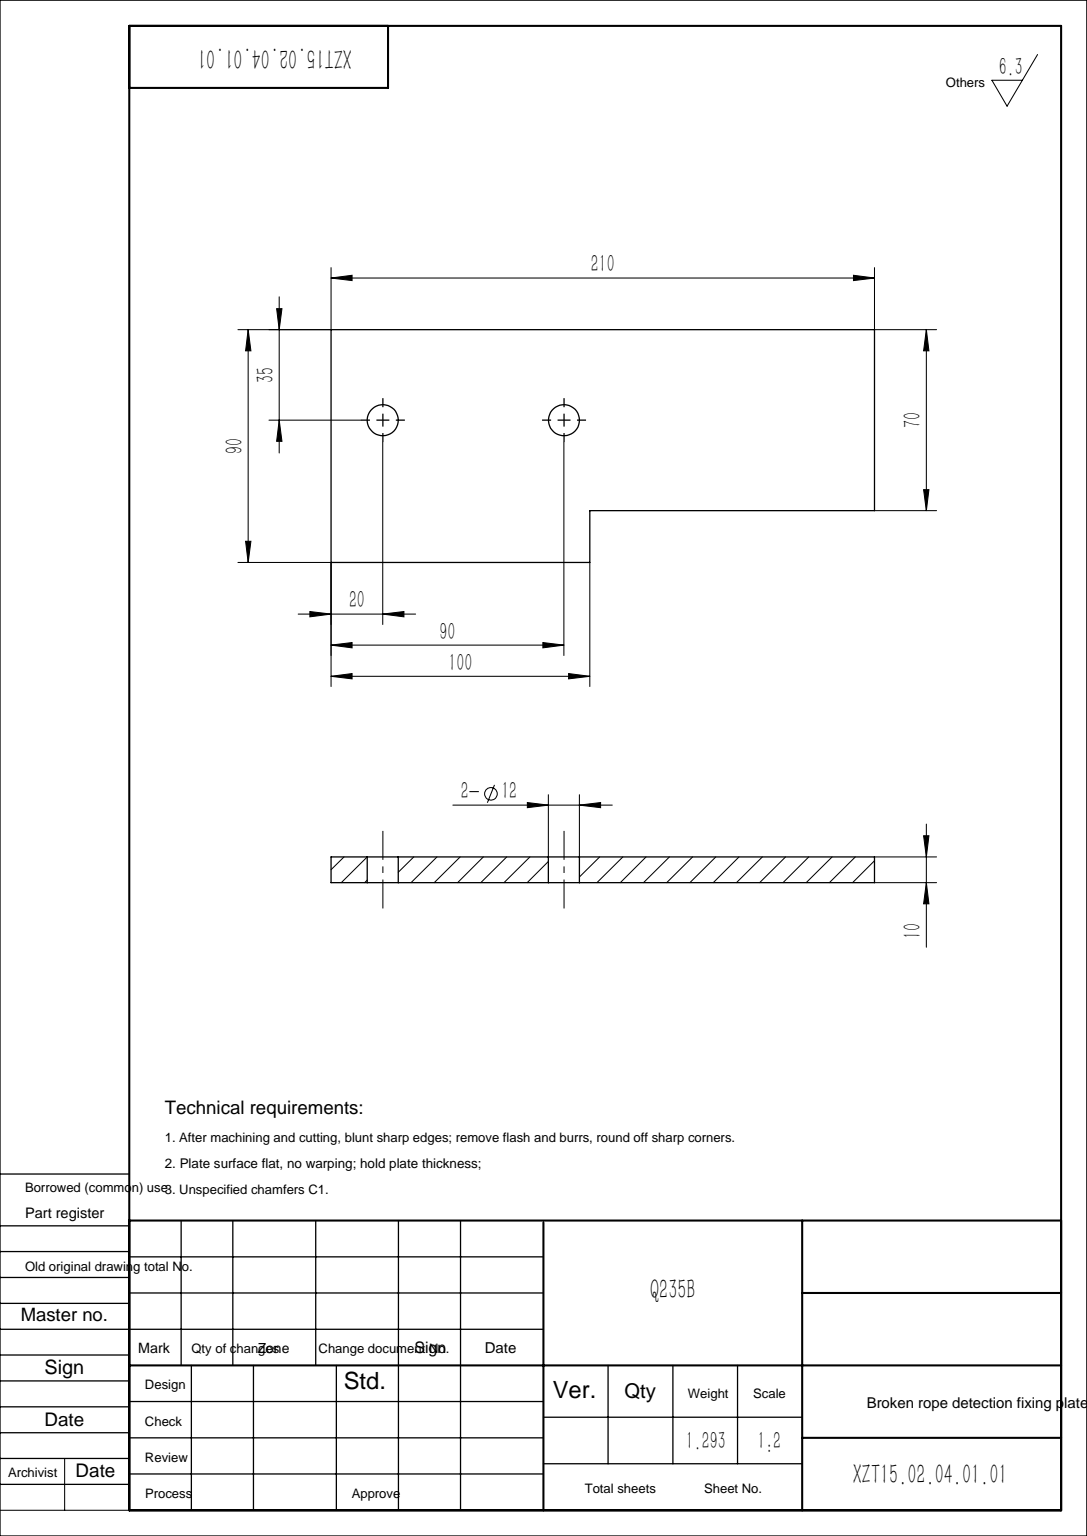
SolidWorks part; units mm, degrees
material "Q235B"
ref_plane "Front Plane" through (0, 0, 0) normal (0, 0, 1) x (1, 0, 0)
ref_plane "Top Plane" through (0, 0, 0) normal (0, 1, 0) x (1, 0, 0)
ref_plane "Right Plane" through (0, 0, 0) normal (1, 0, 0) x (0, 0, -1)
sketch "Sketch1" plane through (0, 0, 0) normal (0, 0, 1) x (1, 0, 0)
  line L0 (0, 0) -> (0, 90)
  line L1 (0, 90) -> (210, 90)
  line L2 (210, 90) -> (210, 20)
  line L3 (210, 20) -> (100, 20)
  line L4 (100, 20) -> (100, 0)
  line L5 (100, 0) -> (0, 0)
  dimension "D1" = 100
  dimension "D2" = 70
  dimension "D3" = 210
  dimension "D4" = 90
extrude "Boss-Extrude1" add sketch "Sketch1" along normal mid plane 10
hole_wizard "Ø12.0 (12) Diameter Hole1" positions "Sketch2" profile "Sketch3" hole size "Ø12.0" standard "GB" end condition up to next
sketch "Sketch2" plane through (0, 0, 5) normal (0, 0, 1) x (1, 0, 0)
  line L0 (210, 90) -> (0, 90) construction
  line L1 (0, 90) -> (0, 0) construction
  point P0 (20, 55)
  point P2 (90, 55)
  dimension "D1" = 35
  dimension "D2" = 20
  dimension "D3" = 90
sketch "Sketch3" plane through (20, 55, 5) normal (1, 0, 0) x (0, -1, 0)
  line L0 (0, 0) -> (0, 10)
  line L1 (0, 10) -> (6, 10)
  line L2 (6, 10) -> (6, 0)
  line L5 (6, 0) -> (0, 0)
  line L11 (0, -6.35) -> (0, 107.95) construction
  dimension "通孔孔直径" = 12
  dimension "通孔孔深度" = 10
